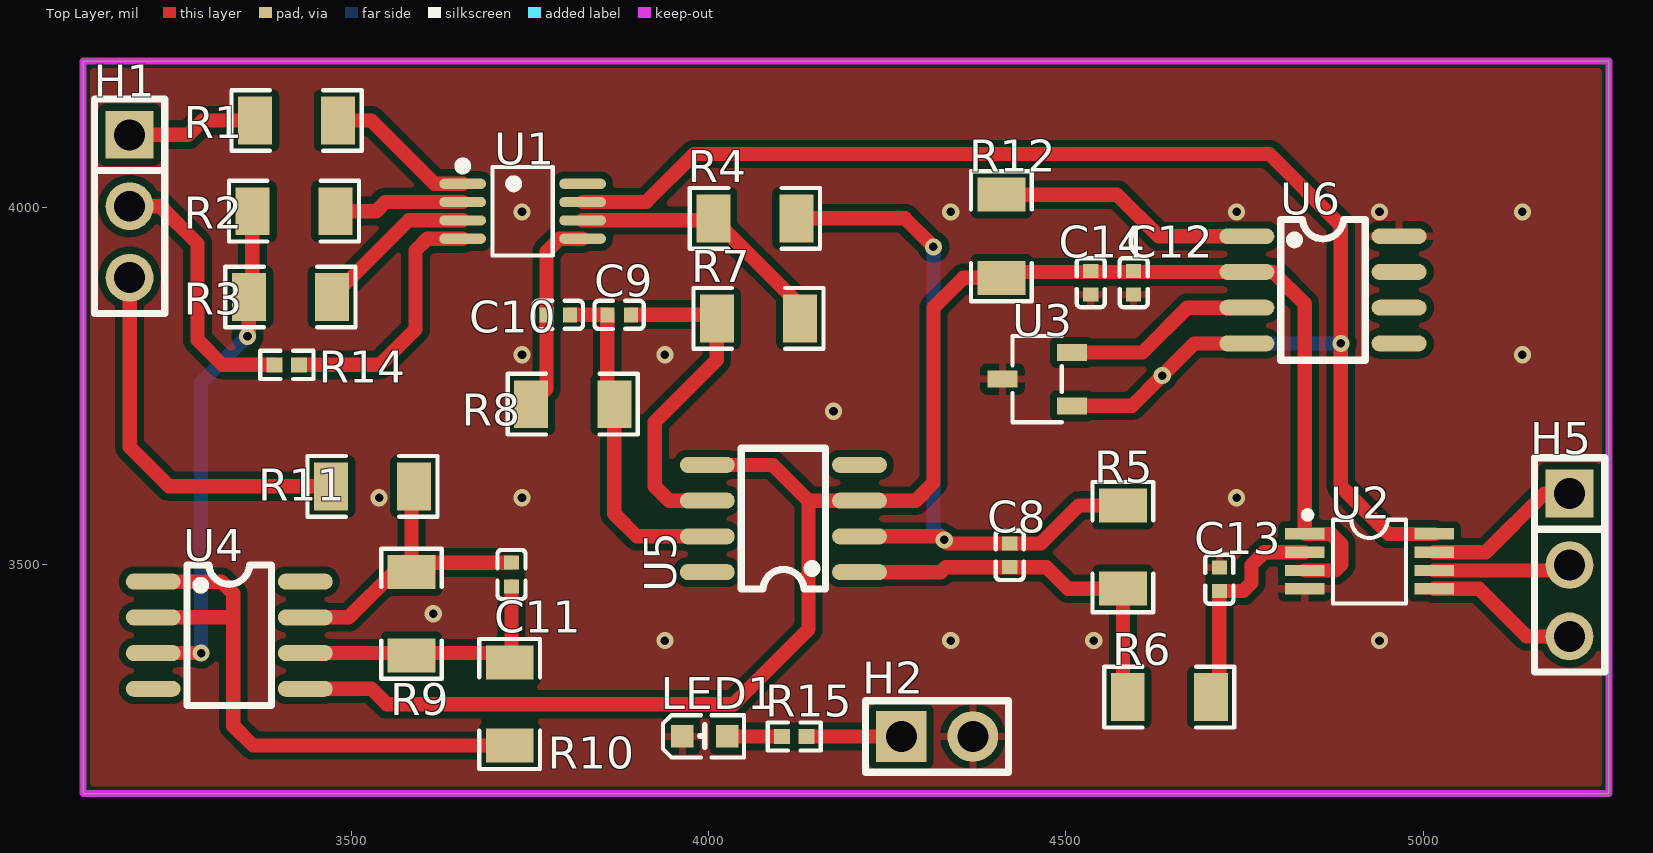
[diagram p0: Top Layer view]
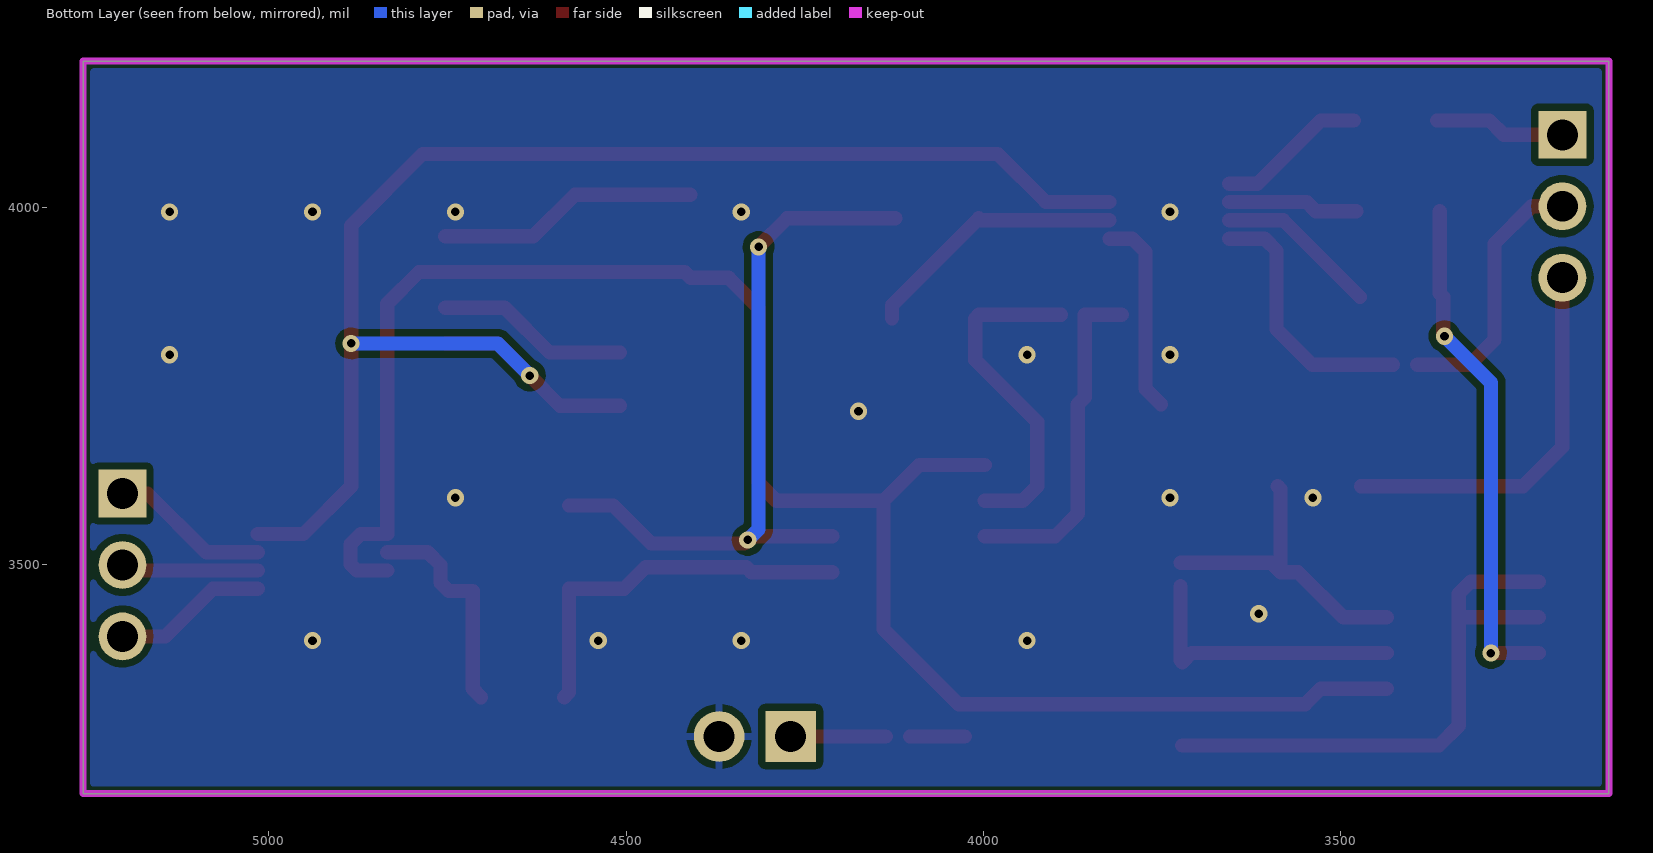
[diagram p1: Bottom Layer view, seen from below]
# Altium PCB MISC52015.pcbdoc
Units mil, origin at the board's own origin, x right, y up, seen from the top; angles counter-clockwise.
Board outline 2135 x 1025 mil, 2 copper layers (Top Layer, Bottom Layer), stack 62.206 mil thick; 31 components, 29 nets, 95 pads, 23 vias.

## Layer stack, top to bottom
Top Solder Mask Layer: solder mask 0.394, Dk 3.3
Top Layer: signal copper 1.379
Dielectric1: surface 59.449, FR4, Dk 4.5
Bottom Layer: signal copper 1.378
Bottom Solder Mask Layer: solder mask 0.394, Dk 3.3

## Board outline
3125,4205 3125,3180 5260,3180 5260,4205

## Design rules (kind name [scope] priority, off if disabled: settings)
BoardOutlineClearance copperThickness2oz_1 [All] p2 off: genericclearance=7.99 ignorepadtopadclearanceinfootprint=FALSE except(0: Arc-SplitContinuation Track-SplitContinuation SMDPad-SplitContinuation THPad-SplitContinuation Via-SplitContinuation Fill-SplitContinuation Region-SplitContinuation Poly-SplitContinuation Text-SplitContinuation Hole-SplitContinuation; 5.98: Arc-CutoutEdge SMDPad-CutoutEdge THPad-CutoutEdge Via-CutoutEdge Fill-CutoutEdge Region-CutoutEdge Text-CutoutEdge; 6.93: Hole-OutlineEdge Hole-CutoutEdge; 10: Poly-OutlineEdge Poly-CutoutEdge; 11.81: Arc-OutlineEdge Track-OutlineEdge SMDPad-OutlineEdge THPad-OutlineEdge Via-OutlineEdge Fill-OutlineEdge Region-OutlineEdge Text-OutlineEdge Track-CutoutEdge)
BoardOutlineClearance copperThickness1oz_1 [All] p4: genericclearance=4.02 ignorepadtopadclearanceinfootprint=FALSE except(0: Arc-SplitContinuation Track-SplitContinuation SMDPad-SplitContinuation THPad-SplitContinuation Via-SplitContinuation Fill-SplitContinuation Region-SplitContinuation Poly-SplitContinuation Text-SplitContinuation Hole-SplitContinuation; 6: SMDPad-CutoutEdge THPad-CutoutEdge Via-CutoutEdge Fill-CutoutEdge Region-CutoutEdge Text-CutoutEdge; 6.93: Hole-OutlineEdge Hole-CutoutEdge; 10: Poly-OutlineEdge Poly-CutoutEdge; 11.8: Arc-OutlineEdge Track-OutlineEdge SMDPad-OutlineEdge THPad-OutlineEdge Via-OutlineEdge Fill-OutlineEdge Region-OutlineEdge Text-OutlineEdge; 11.81: Arc-CutoutEdge Track-CutoutEdge)
Clearance copperThickness2oz [All] p1 off: gap=7.99 ignorepadtopadclearanceinfootprint=FALSE except(5.98: SMDPad-Track SMDPad-SMDPad THPad-Track SMDPad-THPad THPad-THPad Track-Via SMDPad-Via THPad-Via Via-Via Fill-Track Region-Track Fill-SMDPad Region-SMDPad Fill-THPad Region-THPad Fill-Via Region-Via Fill-Fill Fill-Region Region-Region Arc-Track Arc-SMDPad Arc-THPad Arc-Via Fill-Arc Region-Arc Arc-Arc Text-Track SMDPad-Text Text-THPad Text-Via Fill-Text Region-Text Arc-Text Text-Text; 6.93: Hole-Track Hole-SMDPad Hole-THPad Hole-Via Fill-Hole Region-Hole Hole-Arc Hole-Text; 10: Poly-Track Poly-SMDPad Poly-THPad Poly-Via Poly-Fill Poly-Region Poly-Poly Poly-Arc Poly-Text Poly-Hole)
Clearance copperThickness1oz [All] p3: gap=4.02 ignorepadtopadclearanceinfootprint=FALSE except(5.98: SMDPad-Track SMDPad-SMDPad THPad-Track SMDPad-THPad THPad-THPad Track-Via SMDPad-Via THPad-Via Via-Via Fill-Track Region-Track Fill-SMDPad Region-SMDPad Fill-THPad Region-THPad Fill-Via Region-Via Fill-Fill Fill-Region Region-Region; 6: Arc-Track Arc-SMDPad Arc-THPad Arc-Via Fill-Arc Region-Arc Arc-Arc Text-Track SMDPad-Text Text-THPad Text-Via Fill-Text Region-Text Arc-Text Text-Text; 6.93: Hole-Track Hole-SMDPad Hole-THPad Hole-Via Fill-Hole Region-Hole Hole-Arc Hole-Text; 10: Poly-Track Poly-SMDPad Poly-THPad Poly-Via Poly-Fill Poly-Region Poly-Poly Poly-Arc Poly-Text Poly-Hole)
DiffPairsRouting differentialPair [All] p1: maxlimit=6 minlimit=6 mostfreqgap=6 toplayer_minwidth=5 toplayer_prefwidth=10 toplayer_maxwidth=100 toplayer_mingap=6 toplayer_prefgap=6 toplayer_maxgap=6 bottomlayer_minwidth=5 bottomlayer_prefwidth=10 bottomlayer_maxwidth=100 bottomlayer_mingap=6 bottomlayer_prefgap=6 bottomlayer_maxgap=6 maxuncoupledlength=10
HoleToHoleClearance otherClearance [All] p1: gap=11.81 allowstackedmicrovias=TRUE
Length netLength [All] p1: minlimit=0 maxlimit=0
MatchedLengths netLengthTolerance [All] p1: tolerance=1000
PasteMaskExpansion pasteMaskExpansion [All] p1: expansion=0
PlaneConnect innerPlane [All] p1: planeconnectstyle=Relief reliefexpansion=20 reliefentries=4 reliefconductorwidth=10 reliefairgap=10
PolygonConnect copperRegion [(InNet('GND'))] p1: connectstyle=Relief reliefconductorwidth=10 reliefentries=4 polygonreliefangle="90 Angle" airgapwidth=10 via.connectstyle=Relief via.reliefconductorwidth=10 via.reliefentries=4 via.polygonreliefangle="90 Angle" via.airgapwidth=10
RoutingVias viaSize [All] p1: holewidth=12.01 width=24.02 viastyle="Through Hole" minholewidth=11.81 minwidth=19.68 maxholewidth=248.03 maxwidth=393.7
SolderMaskExpansion solderMaskExpansion [IsVia] p1: expansion=-1000 istentingtop=TRUE
SolderMaskExpansion solderMaskExpansion [All] p2: expansion=2 istentingtop=FALSE
Width copperThickness2oz_2 [All] p1 off: maxlimit=100 minlimit=8 preferedwidth=10
Width copperThickness1oz_2 [All] p2: maxlimit=100 minlimit=5 preferedwidth=10

## Components (designator, comment, footprint, x,y, rotation, side; value= is the part's Value field where it differs from the comment)
C8 "0.0015uF" C0402 4421.54,3513.46 r270 top
C9 "1uF" C0402 3875,3850 r0 top
C10 "750pF" C0402 3790,3850 r0 top
C11 "39pF" C0402 3724.45,3486.68 r270 top
C12 "0.1uF" C0402 4595,3895 r90 top
C13 "0.1uF" C0402 4715,3480 r270 top
C14 "10uF" C0402 4535,3895 r270 top
H1 "" HDR-TH_3P-P2.54-V-M 3190,4001.99 r270 top
H2 "" HDR-TH_2P-P2.54-V-M-1 4320,3260 r0 top
H5 "" HDR-TH_3P-P2.54-V-M 5205,3500 r270 top
LED1 "KT-0603W" LED0603-R-RD_WHITE 3995,3260 r0 top
R1 "390kΩ" R1206 3423.67,4121.99 r0 top
R2 "40kΩ" R1206 3420,3995 r0 top
R3 "40kΩ" R1206 3415,3875 r0 top
R4 "5kΩ" R1206 4065,3985 r0 top
R5 "1MΩ" R1206 4580,3525 r270 top
R6 "100Ω" R1206 4645,3315 r0 top
R7 "3.2MΩ" R1206 4070,3845 r0 top
R8 "200kΩ" R1206 3810,3725 r0 top
R9 "390kΩ" R1206 3584.45,3431.68 r270 top
R10 "20kΩ" R1206 3721.87,3305.55 r270 top
R11 "390kΩ" R1206 3530,3610 r0 top
R12 "100Ω" R1206 4410,3960 r270 top
R14 "390kΩ" R0402 3410,3780 r0 top
R15 "1.15kΩ" R0402 4120,3260 r0 top
U1 "INA326EA/2K5" VSSOP-8_L3.0-W3.0-P0.65-LS5.0-BL 3740,3995 r270 top
U2 "ADS8321E/2K5" MSOP-8_L3.0-W3.0-P0.65-LS4.9-BL 4925,3505 r270 top
U3 "REF3125AIDBZR" SOT-23-3_L2.9-W1.6-P1.90-LS2.8-BR 4460,3760 r0 top
U4 "OPA2335AIDR" SOIC-8_L5.0-W4.0-P1.27-LS6.0-BL 3329.45,3401.68 r270 top
U5 "OPA2335AIDR" SOIC-8_L5.0-W4.0-P1.27-LS6.0-BL 4105,3565 r90 top
U6 "OPA2335AIDR" SOIC-8_L5.0-W4.0-P1.27-LS6.0-BL 4860,3885 r270 top

## Footprints (in the part's own frame and the unit in brackets; to place one, negate y for a bottom-side part, rotate by r counter-clockwise, add the part's x,y. Pads: shape width x height; smd on the part's side, far side on the other; paste and mask are expansions set on the pad)
C0402 [mm]
  rect 0.5x0.54 smd: 1(-0.42,0) 2(0.42,0)
  silkscreen extent -0.87,-0.5 0.87,0.5
HDR-TH_2P-P2.54-V-M-1 [mm]
  rect 1.8x1.8 hole 1.1: 1(-1.27,0)
  round 1.8 hole 1.1: 2(1.27,0)
  silkscreen extent -2.54,-1.27 2.54,1.27
HDR-TH_3P-P2.54-V-M [mm]
  rect 1.7x1.7 hole 1.1: 1(-2.54,0)
  round 1.7 hole 1.1: 2(0,0) 3(2.54,0)
  silkscreen extent -3.81,-1.25 3.81,1.25
LED0603-R-RD_WHITE [mm]
  rect 0.8x0.8 smd: 1(0.8,0) 2(-0.8,0)
  silkscreen extent -1.49,-0.75 1.39,0.76
MSOP-8_L3.0-W3.0-P0.65-LS4.9-BL [mil]
  rect 15.98x55 smd: 1(-38.39,-90.55) 2(-12.8,-90.55) 3(12.8,-90.55) 4(38.39,-90.55) 5(38.39,90.55) 6(12.8,90.55) 7(-12.8,90.55) 8(-38.39,90.55)
  silkscreen extent -70,-91 59,51
R0402 [mm]
  rect 0.566x0.54 smd paste-100 mask+0.051: 1(-0.433,0) 2(0.433,0)
  silkscreen extent -0.94,-0.5 0.94,0.5
R1206 [mil]
  rect 47.54x66.97 smd paste-3937.01 mask+2: 1(-58.22,0) 2(58.22,0)
  silkscreen extent -91,-42 91,42
SOIC-8_L5.0-W4.0-P1.27-LS6.0-BL [mil]
  oval 22.38x76.78 smd: 1(-75,-106.5) 2(-25,-106.5) 3(25,-106.5) 4(75,-106.5) 5(75,106.5) 6(25,106.5) 7(-25,106.5) 8(-75,106.5)
  silkscreen extent -98,-59 98,59
SOT-23-3_L2.9-W1.6-P1.90-LS2.8-BR [mm]
  rect 1.07x0.6 smd: 1(1.235,-0.95) 2(1.235,0.95) 3(-1.235,0)
  silkscreen extent -0.88,-1.54 0.88,1.54
VSSOP-8_L3.0-W3.0-P0.65-LS5.0-BL [mil]
  oval 14.33x65.43 smd: 1(-38.39,-83.9) 2(-12.79,-83.9) 3(12.8,-83.9) 4(38.39,-83.9) 5(38.39,83.9) 6(12.8,83.9) 7(-12.79,83.9) 8(-38.39,83.9)
  silkscreen extent -69,-90 62,42

## Via types
v1: diameter 24.02, hole 12, Top Layer to Bottom Layer, 23 vias

## Nets (pads, with @x,y where several pads share a name; then routed paths per layer and width w, separated by ;. In a path a pad name is that pad's centre, name@x,y a point inside that pad or via, vN(x,y) a via of type N, cw(c..) or ccw(c..) an arc to the next point about the centre after c; other vN are vias at no path point)
$1N1: R1.2 U1.1 | length 210.9
  Top Layer w20: R1.2 3528.01,4121.99 3616.61,4033.39 U1.1
$1N2: R2.2 U1.2 | length 183.2
  Top Layer w20: R2.2 3535,3995 3547.79,4007.79 U1.2
$1N3: R3.2 U1.3 | length 227.3
  Top Layer w20: R3.2 3580.42,3982.2 U1.3
$1N6: R10.2 U4.1 U4.2 | length 814.9
  Top Layer w20: U4.2 3333.57,3426.68 3335,3425.25 ; U4.1 3318.32,3476.68 3335,3460 3335,3425.25 ; R10.2 3362.67,3247.33 3335,3275 3335,3425.25
$1N8: R4.1 R7.2 U1.6 | length 374.3
  Top Layer w20: U1.6 4003.98,3982.2 R4.1 4128.22,3863.56 R7.2
$1N9: C8.1 R4.2 R5.1 U5.2 | length 1019.2
  Top Layer w20: R4.2 4275,3985 v1(4314.86,3945.14) ; U5.2 4325,3540 4335,3530 C8.1 4465,3530 4518.22,3583.22 R5.1
  Bottom Layer w20: v1(4314.86,3945.14) 4314.86,3550.14 v1(4330,3535)
$1N10: C13.2 R6.2 U2.2 | length 309.9
  Top Layer w20: R6.2 4715,3326.78 C13.2 4748.46,3463.46 4760,3475 4760,3500 4777.8,3517.8 U2.2
$1N11: C8.2 R5.2 R6.1 U5.1 | length 538.4
  Top Layer w20: U5.1 4325,3490 4331.92,3496.92 C8.2 4473.08,3496.92 4503.22,3466.78 R5.2 4580,3321.78 R6.1
$1N16: C9.2 R7.1 U5.6 | length 475
  Top Layer w20: C9.2 4006.78,3850 R7.1 4011.78,3786.78 3925,3700 3925,3610 3945,3590 U5.6
$1N17: C9.1 C10.2 R8.2 U5.7 | length 477.6
  Top Layer w20: C10.2 C9.1 3858.46,3734.76 R8.2 3868.22,3571.78 3900,3540 U5.7
$1N18: C10.1 R8.1 U1.5 | length 280.4
  Top Layer w20: R8.1 3773.46,3746.68 C10.1 3773.46,3938.46 3791.61,3956.61 U1.5
$1N19: C11.2 R9.2 R10.1 U4.6 | length 398.7
  Top Layer w20: U4.6 3708.96,3376.68 R10.1 3724.45,3366.35 C11.2
$1N20: C11.1 R9.1 R11.2 U4.7 | length 441.9
  Top Layer w20: U4.7 3496.68,3426.68 3559.9,3489.9 R9.1 ; R11.2 3584.45,3606.23 R9.1 ; C11.1 3597.77,3503.22 R9.1
$1N21: H1.3 R11.1 | length 541.5
  Top Layer w20: H1.3 3190,3665 3245,3610 R11.1
$1N23: R12.1 U6.1 | length 367.6
  Top Layer w20: R12.1 4571.78,4018.22 4630,3960 U6.1
$1N27: U3.2 U6.3 | length 270.8
  Top Layer w20: U3.2 4607.4,3797.4 4670,3860 U6.3
$1N34: R14.2 U1.4 | length 366.7
  Top Layer w20: R14.2 3540,3780 3590,3830 3590,3940 3606.61,3956.61 U1.4
$1N37: U1.8
$1N41: R2.1 R3.1 U4.3 | length 715.1
  Top Layer w20: U4.3 v1(3290,3376.68) ; v1(3355,3820) 3356.78,3821.78 R3.1 3361.78,3880 R2.1
  Bottom Layer w20: v1(3290,3376.68) 3290,3755 v1(3355,3820)
$1N47: H1.1 R1.1 | length 183.7
  Top Layer w20: H1.1 3271.99,4101.99 3291.99,4121.99 R1.1
$1N48: H1.2 R14.1 | length 374
  Top Layer w20: H1.2 3233.01,4001.99 3285,3950 3285,3815 3320,3780 R14.1
$1N49: H5.1 U2.7 | length 223.5
  Top Layer w20: U2.7 5087.8,3517.8 5170,3600 H5.1
$1N50: H5.2 U2.6 | length 192.7
  Top Layer w20: U2.6 5197.2,3492.2 H5.2
$1N51: H5.3 U2.5 | length 217
  Top Layer w20: U2.5 5078.39,3466.61 5145,3400 H5.3
$1N52: H2.1 R15.2 | length 133
  Top Layer w20: R15.2 H2.1
$1N53: LED1.1 R15.1 | length 76.5
  Top Layer w20: LED1.1 R15.1
+2.5V: C12.2 C14.1 R12.2 U2.1 U2.3 U4.5 U5.3 U5.5 U6.2 | length 2550.4
  Top Layer w20: U4.5 3528.32,3326.68 3550,3305 4035,3305 4140,3410 4140,3590 ; U5.5 4090,3640 4140,3590 ; U2.3 4877.2,3492.2 4885.86,3500.86 4885.86,3529.14 4871.61,3543.39 U2.1 4834.45,3865.55 4790,3910 U6.2 4418.22,3910 R12.2 4356.78,3901.78 4315,3860 4315,3615 4290,3590 U5.3 4140,3590
+5V: U1.7 U2.8 U3.1 U6.4 | length 2203.2
  Top Layer w20: U1.7 3912.79,4007.79 3980,4075 4785,4075 4885,3975 v1(4885,3810) 4885,3610 4951.61,3543.39 U2.8 ; U3.1 4592.6,3722.6 v1(4635,3765) 4680,3810 U6.4
  Bottom Layer w20: v1(4635,3765) 4680,3810 v1(4885,3810)
GND: C12.1 C13.1 C14.2 H2.2 LED1.2 U2.4 U3.3 U6.8
  other v1: 3939.1,3394.1 4339.1,3394.1 4539.1,3394.1 4939.1,3394.1 3614.91,3431.68 3539.1,3594.1 3739.1,3594.1 4739.1,3594.1 4175,3715 3739.1,3794.1 3939.1,3794.1 5139.1,3794.1 3739.1,3994.1 4339.1,3994.1 4739.1,3994.1 4939.1,3994.1 5139.1,3994.1
pads on no net: U4.4 U4.8 U5.4 U5.8 U6.5 U6.6 U6.7

## Polygon pours and split planes (outlines as drawn)
GND on Top Layer (solid, remove dead copper, pour order 0): 3000,4350 3000,3000 5480,3000 5480,4350
GND on Bottom Layer (solid, remove dead copper, pour order 2): 3040,4285 3040,3000 5430,3000 5430,4285

## Keep-outs
Board Outline Layer:
  the board outline again, w10